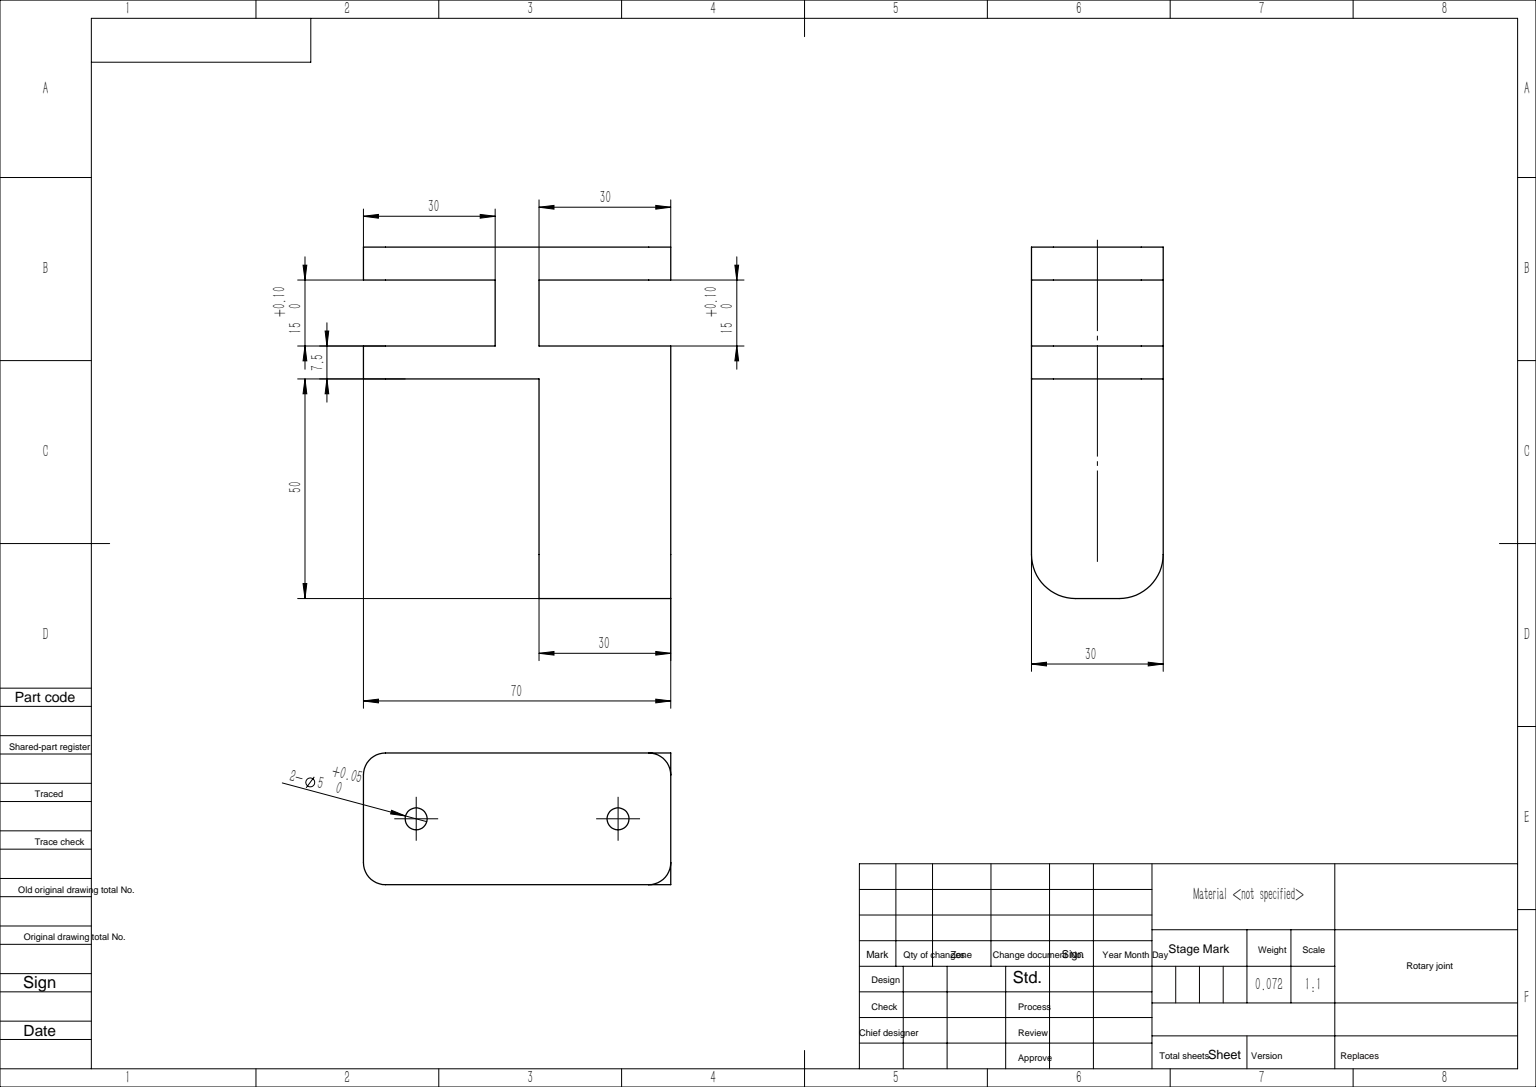
SolidWorks part; units mm, degrees
ref_plane "Front Plane" through (0, 0, 0) normal (0, 0, 1) x (1, 0, 0)
ref_plane "Top Plane" through (0, 0, 0) normal (0, 1, 0) x (1, 0, 0)
ref_plane "Right Plane" through (0, 0, 0) normal (1, 0, 0) x (0, 0, -1)
sketch "Sketch1" plane through (0, 0, 0) normal (0, 0, 1) x (1, 0, 0)
  line L0 (0, 0) -> (0, 70)
  line L1 (0, 70) -> (30, 70)
  line L2 (30, 70) -> (30, 30)
  line L3 (30, 30) -> (80, 30)
  line L4 (80, 30) -> (80, 0)
  line L5 (80, 0) -> (0, 0)
  dimension "D1" = 30
  dimension "D2" = 30
  dimension "D3" = 80
  dimension "D4" = 70
extrude "Boss-Extrude1" add sketch "Sketch1" along normal blind 30
sketch "Sketch4" plane through (0, 0, 0) normal (0, -1, 0) x (-1, 0, 0)
  line L0 (-80, -30) -> (-80, 0) construction
  circle A0 centre (-65, -15) radius 9
  dimension "D1" = 18
  dimension "D2" = 15
extrude "Cut-Extrude2" cut sketch "Sketch4" against normal blind 25
sketch "Sketch5" plane through (0, 0, 0) normal (0, 0, -1) x (-1, 0, 0)
  line L0 (-30, 70) -> (0, 70) construction
  line L1 (-7.5, 70) -> (-22.5, 70)
  line L2 (-7.5, 70) -> (-7.5, 40)
  line L3 (-7.5, 40) -> (-22.5, 40)
  line L4 (-22.5, 70) -> (-22.5, 40)
  line L5 (-30, 30) -> (-30, 70) construction
  line L6 (0, 0) -> (-80, 0) construction
  line L7 (-7.5, 30) -> (-22.5, 30)
  line L8 (-7.5, 30) -> (-7.5, 0)
  line L9 (-7.5, 0) -> (-22.5, 0)
  line L10 (-22.5, 30) -> (-22.5, 0)
  dimension "D1" = 30
  dimension "D2" = 15
  dimension "D3" = 7.5
  dimension "D4" = 30
extrude "Cut-Extrude3" cut sketch "Sketch5" against normal through all
sketch "Sketch6" plane through (22.5, 0, 0) normal (-1, 0, 0) x (0, 0, 1)
  line L0 (30, 70) -> (0, 70) construction
  line L1 (0, 30) -> (0, 0) construction
  line L2 (30, 0) -> (0, 0) construction
  circle A0 centre (15, 58) radius 2.5
  circle A1 centre (15, 12) radius 2.5
  dimension "D1" = 5
  dimension "D3" = 15
  dimension "D4" = 5
  dimension "D5" = 12
  dimension "D2" = 12
extrude "Cut-Extrude4" cut sketch "Sketch6" against normal mid plane 50
fillet "Fillet1" radius 5 6 edges at (3.75, 0, 30) (3.75, 0, 0) (26.25, 70, 30) (3.75, 70, 30) (26.25, 70, 0) (3.75, 70, 0)
fillet "Fillet2" radius 10 2 edges at (80, 15, 0) (80, 15, 30)
